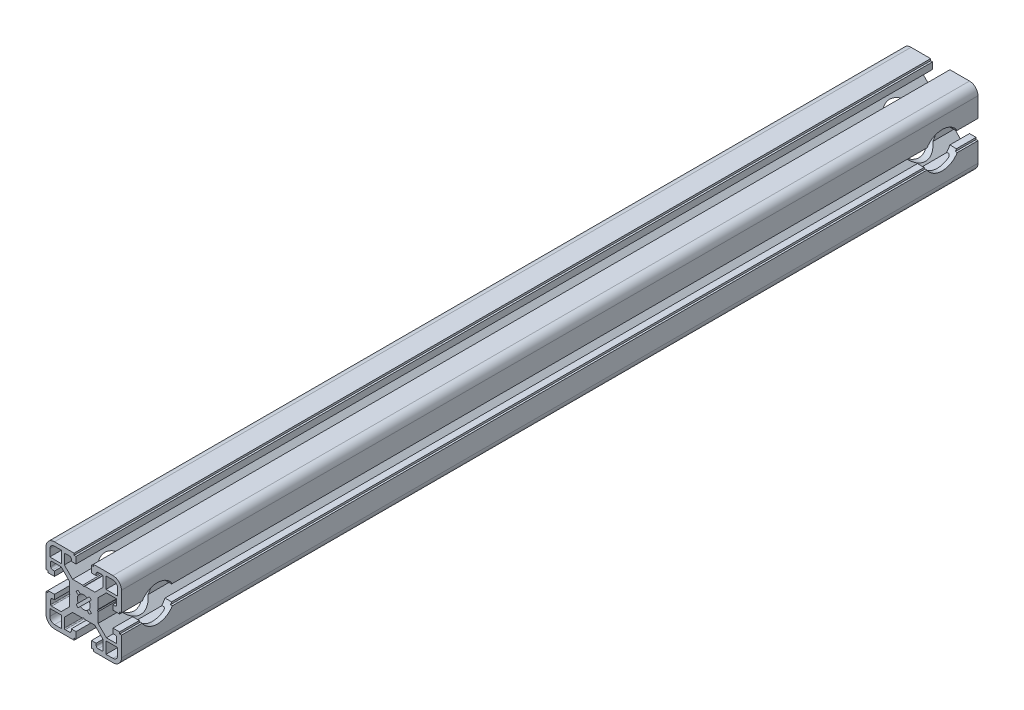
from build123d import *

# Parameters (mm, degrees)
EXTRUDE_1_DEPTH         = 454
HOLE_WIZARD_19_0_19_1_D = 19


with BuildPart() as part:
    # 草图1 → 凸台-拉伸1 (new body)
    with BuildSketch(Plane.XY):
        with BuildLine():
            Line((-18.9995, -4.100341675), (-18.9995, -5.100341675))
            Line((-18.9995, -5.100341675), (-19.9995, -5.100341675))
            Line((-19.9995, -5.100341675), (-19.9995, -15.500341675))
            ThreePointArc((-19.9995, -15.500341675), (-18.681480515, -18.682322191), (-15.4995, -20.000341675))
            Line((-15.4995, -20.000341675), (-5.0995, -20.000341675))
            Line((-5.0995, -20.000341675), (-5.0995, -19.000341675))
            Line((-5.0995, -19.000341675), (-4.0995, -19.000341675))
            Line((-4.0995, -19.000341675), (-4.0995, -15.500341675))
            Line((-4.0995, -15.500341675), (-6.5995, -15.500341675))
            Line((-6.5995, -15.500341675), (-6.5995, -16.500341675))
            ThreePointArc((-6.5995, -16.500341675), (-6.892393219, -17.207448457), (-7.5995, -17.500341675))
            Line((-7.5995, -17.500341675), (-9.7995, -17.500341675))
            ThreePointArc((-9.7995, -17.500341675), (-10.153053391, -17.353895066), (-10.2995, -17.000341675))
            Line((-10.2995, -17.000341675), (-10.2995, -11.997341675))
            Line((-10.2995, -11.997341675), (-5.9025, -7.600341675))
            Line((-5.9025, -7.600341675), (-0.5195, -7.600341675))
            Line((-0.5195, -7.600341675), (0.0005, -7.300341675))
            Line((0.0005, -7.300341675), (0.5195, -7.600341675))
            Line((0.5195, -7.600341675), (5.9035, -7.600341675))
            Line((5.9035, -7.600341675), (10.3005, -11.997341675))
            Line((10.3005, -11.997341675), (10.3005, -17.000341675))
            ThreePointArc((10.3005, -17.000341675), (10.154053391, -17.353895066), (9.8005, -17.500341675))
            Line((9.8005, -17.500341675), (7.6005, -17.500341675))
            ThreePointArc((7.6005, -17.500341675), (6.893393219, -17.207448457), (6.6005, -16.500341675))
            Line((6.6005, -16.500341675), (6.6005, -15.500341675))
            Line((6.6005, -15.500341675), (4.1005, -15.500341675))
            Line((4.1005, -15.500341675), (4.1005, -19.000341675))
            Line((4.1005, -19.000341675), (5.1005, -19.000341675))
            Line((5.1005, -19.000341675), (5.1005, -20.000341675))
            Line((5.1005, -20.000341675), (15.5005, -20.000341675))
            ThreePointArc((15.5005, -20.000341675), (18.682480515, -18.682322191), (20.0005, -15.500341675))
            Line((20.0005, -15.500341675), (20.0005, -5.100341675))
            Line((20.0005, -5.100341675), (19.0005, -5.100341675))
            Line((19.0005, -5.100341675), (19.0005, -4.100341675))
            Line((19.0005, -4.100341675), (15.5005, -4.100341675))
            Line((15.5005, -4.100341675), (15.5005, -6.600341675))
            Line((15.5005, -6.600341675), (16.5005, -6.600341675))
            ThreePointArc((16.5005, -6.600341675), (17.207606781, -6.893234894), (17.5005, -7.600341675))
            Line((17.5005, -7.600341675), (17.5005, -9.800341675))
            ThreePointArc((17.5005, -9.800341675), (17.354053391, -10.153895066), (17.0005, -10.300341675))
            Line((17.0005, -10.300341675), (11.9975, -10.300341675))
            Line((11.9975, -10.300341675), (7.6005, -5.903341675))
            Line((7.6005, -5.903341675), (7.6005, -0.520341675))
            Line((7.6005, -0.520341675), (7.3005, -0.000341675))
            Line((7.3005, -0.000341675), (7.6005, 0.519658325))
            Line((7.6005, 0.519658325), (7.6005, 5.902658325))
            Line((7.6005, 5.902658325), (11.9975, 10.299658325))
            Line((11.9975, 10.299658325), (17.0005, 10.299658325))
            ThreePointArc((17.0005, 10.299658325), (17.354053391, 10.153211715), (17.5005, 9.799658325))
            Line((17.5005, 9.799658325), (17.5005, 7.599658325))
            ThreePointArc((17.5005, 7.599658325), (17.207606781, 6.892551543), (16.5005, 6.599658325))
            Line((16.5005, 6.599658325), (15.5005, 6.599658325))
            Line((15.5005, 6.599658325), (15.5005, 4.099658325))
            Line((15.5005, 4.099658325), (19.0005, 4.099658325))
            Line((19.0005, 4.099658325), (19.0005, 5.099658325))
            Line((19.0005, 5.099658325), (20.0005, 5.099658325))
            Line((20.0005, 5.099658325), (20.0005, 15.499658325))
            ThreePointArc((20.0005, 15.499658325), (18.682480515, 18.68163884), (15.5005, 19.999658325))
            Line((15.5005, 19.999658325), (5.1005, 19.999658325))
            Line((5.1005, 19.999658325), (5.1005, 18.999658325))
            Line((5.1005, 18.999658325), (4.1005, 18.999658325))
            Line((4.1005, 18.999658325), (4.1005, 15.499658325))
            Line((4.1005, 15.499658325), (6.6005, 15.499658325))
            ThreePointArc((6.6005, 15.499658325), (6.393348977, 15.999658325), (6.6005, 16.499658325))
            ThreePointArc((6.6005, 16.499658325), (6.893393219, 17.206765106), (7.6005, 17.499658325))
            Line((7.6005, 17.499658325), (9.8005, 17.499658325))
            ThreePointArc((9.8005, 17.499658325), (10.154053391, 17.353211715), (10.3005, 16.999658325))
            Line((10.3005, 16.999658325), (10.3005, 11.996658325))
            Line((10.3005, 11.996658325), (5.9035, 7.599658325))
            Line((5.9035, 7.599658325), (0.5195, 7.599658325))
            Line((0.5195, 7.599658325), (0.0005, 7.299658325))
            Line((0.0005, 7.299658325), (-0.5195, 7.599658325))
            Line((-0.5195, 7.599658325), (-5.9025, 7.599658325))
            Line((-5.9025, 7.599658325), (-10.2995, 11.996658325))
            Line((-10.2995, 11.996658325), (-10.2995, 16.999658325))
            ThreePointArc((-10.2995, 16.999658325), (-10.153053391, 17.353211715), (-9.7995, 17.499658325))
            Line((-9.7995, 17.499658325), (-7.5995, 17.499658325))
            ThreePointArc((-7.5995, 17.499658325), (-6.892393219, 17.206765106), (-6.5995, 16.499658325))
            Line((-6.5995, 16.499658325), (-6.5995, 15.499658325))
            Line((-6.5995, 15.499658325), (-4.0995, 15.499658325))
            Line((-4.0995, 15.499658325), (-4.0995, 18.999658325))
            Line((-4.0995, 18.999658325), (-5.0995, 18.999658325))
            Line((-5.0995, 18.999658325), (-5.0995, 19.999658325))
            Line((-5.0995, 19.999658325), (-15.4995, 19.999658325))
            ThreePointArc((-15.4995, 19.999658325), (-18.681480515, 18.68163884), (-19.9995, 15.499658325))
            Line((-19.9995, 15.499658325), (-19.9995, 5.099658325))
            Line((-19.9995, 5.099658325), (-18.9995, 5.099658325))
            Line((-18.9995, 5.099658325), (-18.9995, 4.099658325))
            Line((-18.9995, 4.099658325), (-15.4995, 4.099658325))
            Line((-15.4995, 4.099658325), (-15.4995, 6.599658325))
            Line((-15.4995, 6.599658325), (-16.4995, 6.599658325))
            ThreePointArc((-16.4995, 6.599658325), (-17.206606781, 6.892551543), (-17.4995, 7.599658325))
            Line((-17.4995, 7.599658325), (-17.4995, 9.799658325))
            ThreePointArc((-17.4995, 9.799658325), (-17.353053391, 10.153211715), (-16.9995, 10.299658325))
            Line((-16.9995, 10.299658325), (-11.9965, 10.299658325))
            Line((-11.9965, 10.299658325), (-7.5995, 5.902658325))
            Line((-7.5995, 5.902658325), (-7.5995, 0.519658325))
            Line((-7.5995, 0.519658325), (-7.2995, -0.000341675))
            Line((-7.2995, -0.000341675), (-7.5995, -0.520341675))
            Line((-7.5995, -0.520341675), (-7.5995, -5.903341675))
            Line((-7.5995, -5.903341675), (-11.9965, -10.300341675))
            Line((-11.9965, -10.300341675), (-16.9995, -10.300341675))
            ThreePointArc((-16.9995, -10.300341675), (-17.353053391, -10.153895066), (-17.4995, -9.800341675))
            Line((-17.4995, -9.800341675), (-17.4995, -7.600341675))
            ThreePointArc((-17.4995, -7.600341675), (-17.206606781, -6.893234894), (-16.4995, -6.600341675))
            Line((-16.4995, -6.600341675), (-15.4995, -6.600341675))
            Line((-15.4995, -6.600341675), (-15.4995, -4.100341675))
            Line((-15.4995, -4.100341675), (-18.9995, -4.100341675))
        make_face()
        with BuildLine():
            Line((15.5005, -18.000341675), (11.8005, -18.000341675))
            Line((11.8005, -18.000341675), (11.8005, -11.800341675))
            Line((11.8005, -11.800341675), (18.0005, -11.800341675))
            Line((18.0005, -11.800341675), (18.0005, -15.500341675))
            ThreePointArc((18.0005, -15.500341675), (17.268266953, -17.268108628), (15.5005, -18.000341675))
        make_face(mode=Mode.SUBTRACT)
        with BuildLine():
            Line((18.0005, 11.799658325), (11.8005, 11.799658325))
            Line((11.8005, 11.799658325), (11.8005, 17.999658325))
            Line((11.8005, 17.999658325), (15.5005, 17.999658325))
            ThreePointArc((15.5005, 17.999658325), (17.268266953, 17.267425278), (18.0005, 15.499658325))
            Line((18.0005, 15.499658325), (18.0005, 11.799658325))
        make_face(mode=Mode.SUBTRACT)
        with BuildLine():
            Line((-1.8145, -2.875341675), (-3.004391671, -4.066450004))
            Line((-3.004391671, -4.066450004), (-4.065608329, -3.005233346))
            Line((-4.065608329, -3.005233346), (-2.8745, -1.815341675))
            ThreePointArc((-2.8745, -1.815341675), (-3.399473913, -0.000341675), (-2.8745, 1.814658325))
            Line((-2.8745, 1.814658325), (-4.064391671, 3.005766654))
            Line((-4.064391671, 3.005766654), (-3.004391671, 4.065766654))
            Line((-3.004391671, 4.065766654), (-1.8145, 2.874658325))
            ThreePointArc((-1.8145, 2.874658325), (0, 3.399316649), (1.8145, 2.874658325))
            Line((1.8145, 2.874658325), (3.0055, 4.065658325))
            Line((3.0055, 4.065658325), (4.066608329, 3.004549996))
            Line((4.066608329, 3.004549996), (2.8755, 1.814658325))
            ThreePointArc((2.8755, 1.814658325), (3.400473913, -0.000341675), (2.8755, -1.815341675))
            Line((2.8755, -1.815341675), (4.066608329, -3.005233346))
            Line((4.066608329, -3.005233346), (3.0055, -4.066341675))
            Line((3.0055, -4.066341675), (1.8145, -2.875341675))
            ThreePointArc((1.8145, -2.875341675), (0, -3.4), (-1.8145, -2.875341675))
        make_face(mode=Mode.SUBTRACT)
        with BuildLine():
            Line((-17.9995, -15.500341675), (-17.9995, -11.800341675))
            Line((-17.9995, -11.800341675), (-11.7995, -11.800341675))
            Line((-11.7995, -11.800341675), (-11.7995, -18.000341675))
            Line((-11.7995, -18.000341675), (-15.4995, -18.000341675))
            ThreePointArc((-15.4995, -18.000341675), (-17.267266953, -17.268108628), (-17.9995, -15.500341675))
        make_face(mode=Mode.SUBTRACT)
        with BuildLine():
            Line((-11.7995, 17.999658325), (-11.7995, 11.799658325))
            Line((-11.7995, 11.799658325), (-17.9995, 11.799658325))
            Line((-17.9995, 11.799658325), (-17.9995, 15.499658325))
            ThreePointArc((-17.9995, 15.499658325), (-17.267266953, 17.267425278), (-15.4995, 17.999658325))
            Line((-15.4995, 17.999658325), (-11.7995, 17.999658325))
        make_face(mode=Mode.SUBTRACT)
    extrude(amount=-EXTRUDE_1_DEPTH)

    # Ø19.0 (19) 直径孔1 (through all)
    with Locations(Plane(origin=(20.0005, 0, 0), x_dir=(0, 0, -1), z_dir=(1, 0, 0))):
        with Locations((18.999999997, -0.000341675), (435, -0.000341675)):
            Hole(HOLE_WIZARD_19_0_19_1_D / 2)


solid = part.part
